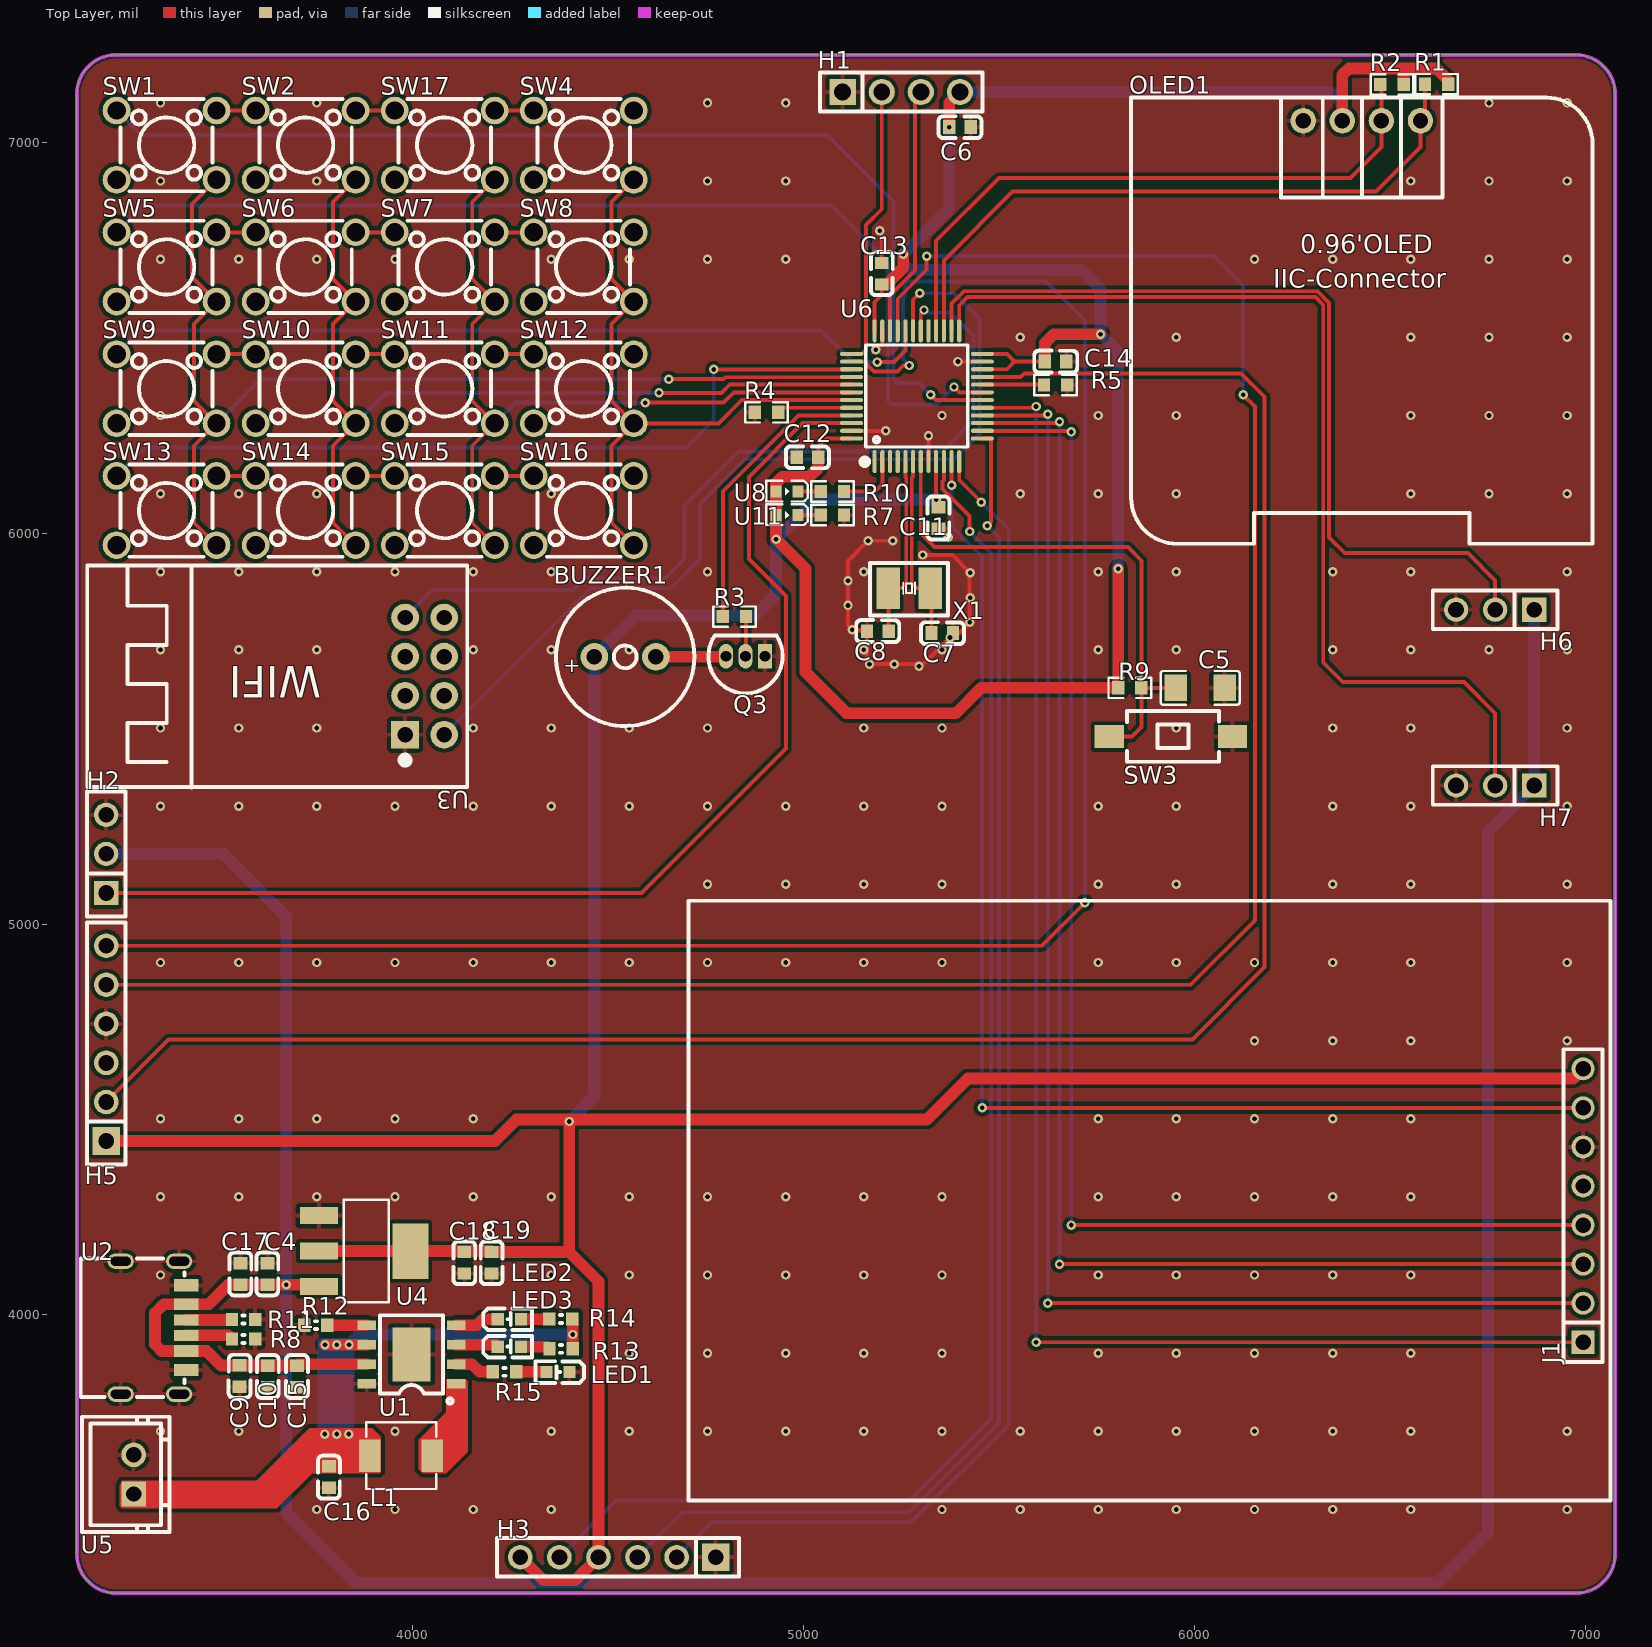
[diagram p0: Top Layer view]
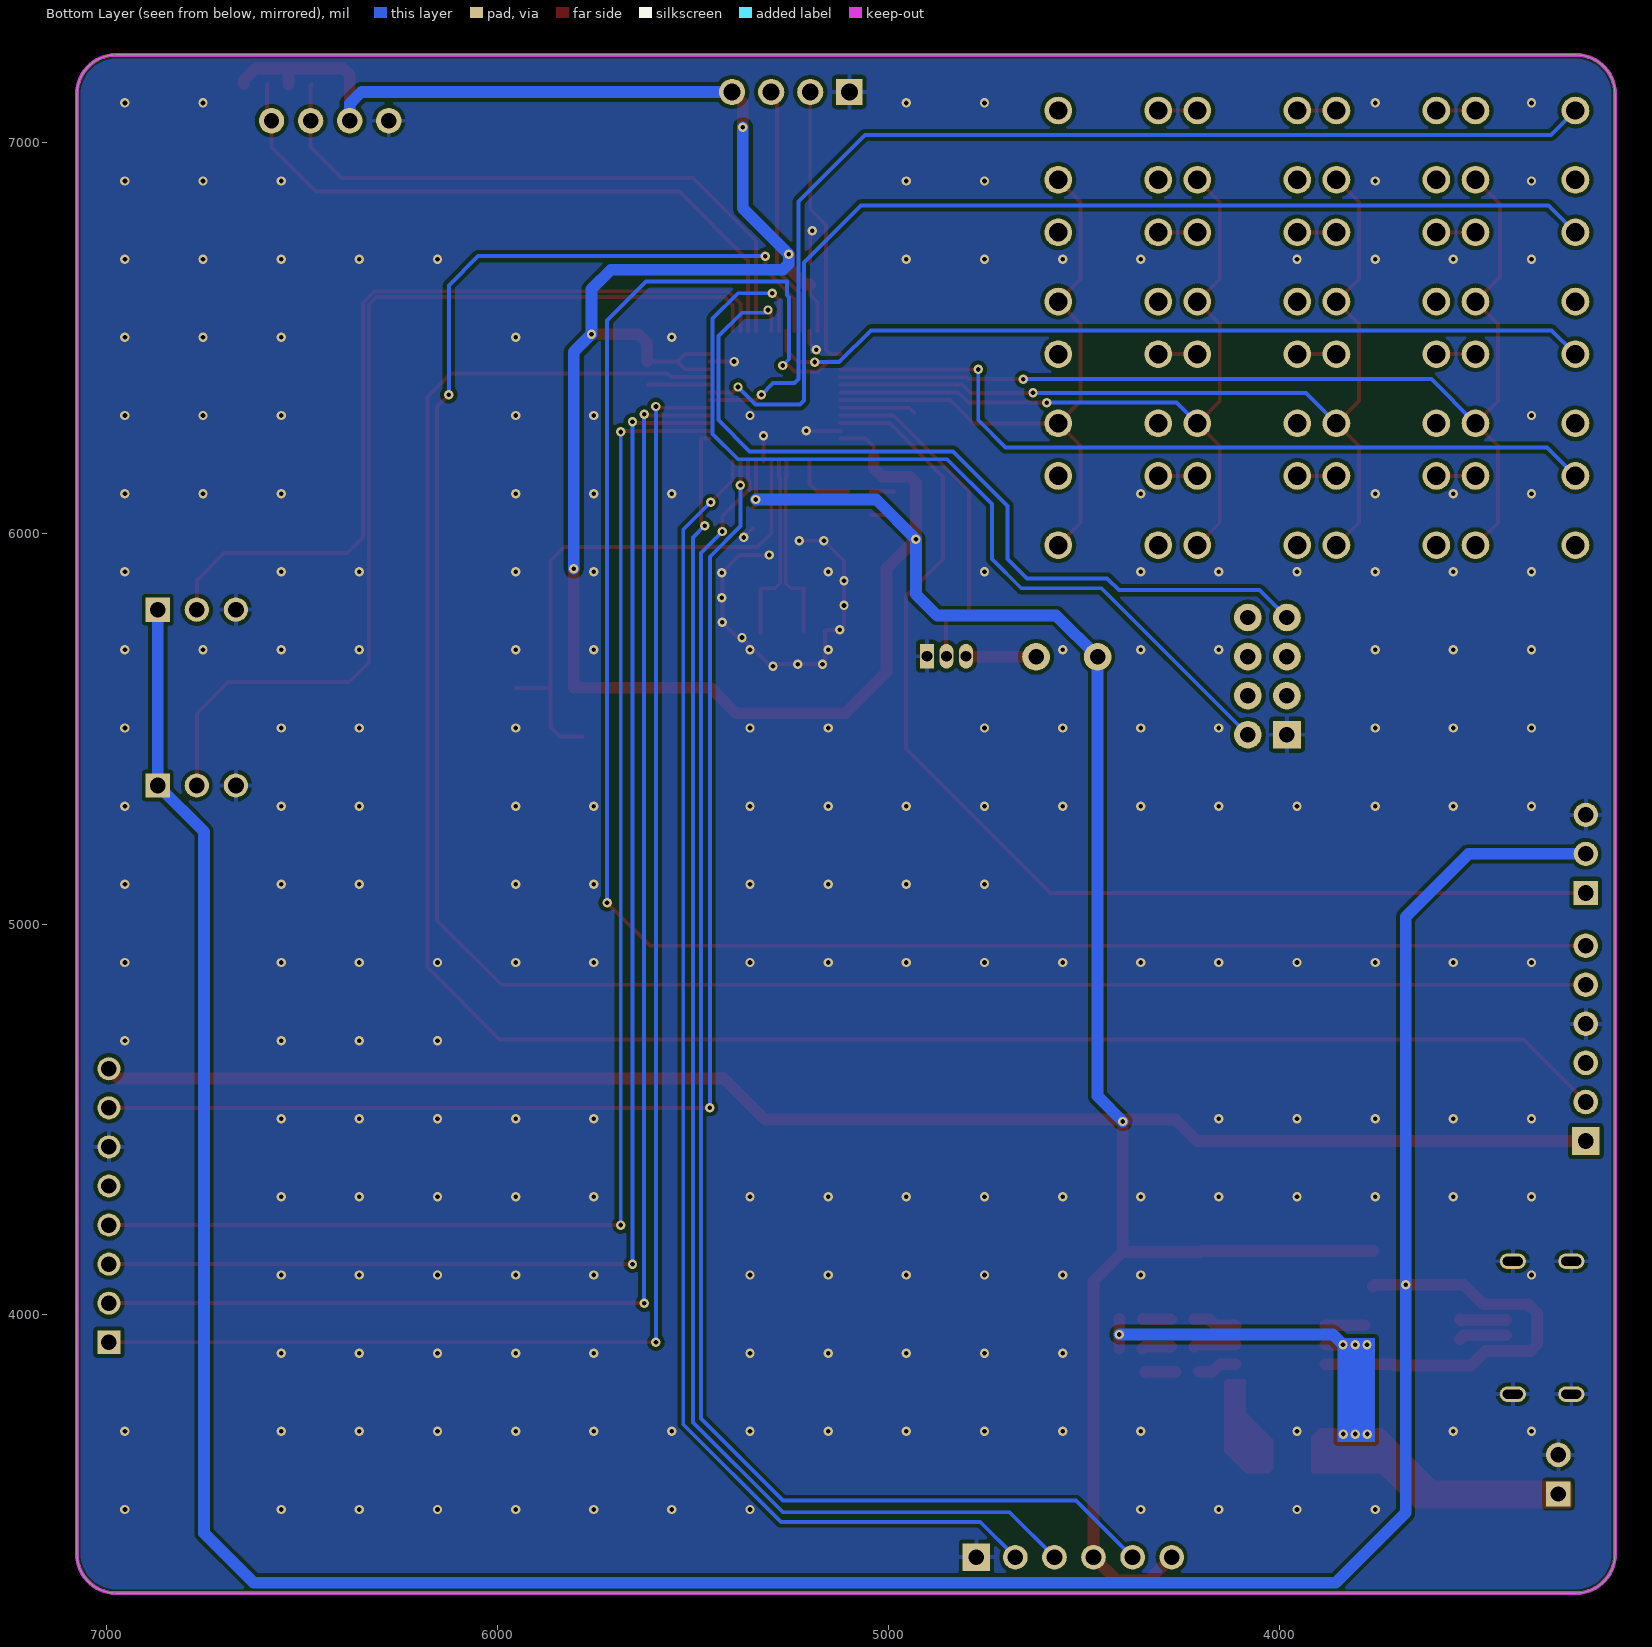
[diagram p1: Bottom Layer view, seen from below]
# Altium PCB MISC51820.pcbdoc
Units mil, origin at the board's own origin, x right, y up, seen from the top; angles counter-clockwise.
Board outline 3937.01 x 3937.01 mil, 2 copper layers (Top Layer, Bottom Layer), stack 62.206 mil thick; 70 components, 71 nets, 263 pads, 270 vias.

## Layer stack, top to bottom
Top Solder Mask Layer: solder mask 0.394, Dk 3.3
Top Layer: signal copper 1.379
Dielectric1: surface 59.449, FR4, Dk 4.5
Bottom Layer: signal copper 1.378
Bottom Solder Mask Layer: solder mask 0.394, Dk 3.3

## Board outline
3240,7225 ccw(c3240,7125) 3140,7125 3140,3387.99 ccw(c3240,3387.99) 3240,3287.99 6977.01,3287.99 ccw(c6977.01,3387.99) 7077.01,3387.99 7077.01,7125 ccw(c6977.01,7125) 6977.01,7225

## Design rules (kind name [scope] priority, off if disabled: settings)
BoardOutlineClearance copperThickness2oz_1 [All] p2 off: genericclearance=7.99 ignorepadtopadclearanceinfootprint=FALSE except(0: Arc-SplitContinuation Track-SplitContinuation SMDPad-SplitContinuation THPad-SplitContinuation Via-SplitContinuation Fill-SplitContinuation Region-SplitContinuation Poly-SplitContinuation Text-SplitContinuation Hole-SplitContinuation; 5.98: Arc-CutoutEdge Track-CutoutEdge SMDPad-CutoutEdge THPad-CutoutEdge Via-CutoutEdge Text-CutoutEdge; 6.9: Hole-OutlineEdge Hole-CutoutEdge; 10: Poly-OutlineEdge Poly-CutoutEdge; 11.81: Arc-OutlineEdge Track-OutlineEdge SMDPad-OutlineEdge THPad-OutlineEdge Via-OutlineEdge Fill-OutlineEdge Region-OutlineEdge Text-OutlineEdge Fill-CutoutEdge Region-CutoutEdge)
BoardOutlineClearance Plane_innerPlane_1 [All] p4 off: genericclearance=4.02 ignorepadtopadclearanceinfootprint=FALSE except(0: Arc-SplitContinuation Track-SplitContinuation SMDPad-SplitContinuation THPad-SplitContinuation Via-SplitContinuation Fill-SplitContinuation Region-SplitContinuation Poly-SplitContinuation Text-SplitContinuation Hole-SplitContinuation; 5.98: Arc-CutoutEdge Track-CutoutEdge SMDPad-CutoutEdge THPad-CutoutEdge Via-CutoutEdge Text-CutoutEdge; 6.9: Hole-OutlineEdge Hole-CutoutEdge; 10: Poly-OutlineEdge Poly-CutoutEdge; 11.81: Arc-OutlineEdge Track-OutlineEdge SMDPad-OutlineEdge THPad-OutlineEdge Via-OutlineEdge Fill-OutlineEdge Region-OutlineEdge Text-OutlineEdge Fill-CutoutEdge Region-CutoutEdge)
BoardOutlineClearance Copper_copperRegion_1 [All] p6 off: genericclearance=4.02 ignorepadtopadclearanceinfootprint=FALSE except(0: Arc-SplitContinuation Track-SplitContinuation SMDPad-SplitContinuation THPad-SplitContinuation Via-SplitContinuation Fill-SplitContinuation Region-SplitContinuation Poly-SplitContinuation Text-SplitContinuation Hole-SplitContinuation; 5.98: Arc-CutoutEdge Track-CutoutEdge SMDPad-CutoutEdge THPad-CutoutEdge Via-CutoutEdge Text-CutoutEdge; 6.9: Hole-OutlineEdge Hole-CutoutEdge; 10: Poly-OutlineEdge Poly-CutoutEdge; 11.81: Arc-OutlineEdge Track-OutlineEdge SMDPad-OutlineEdge THPad-OutlineEdge Via-OutlineEdge Fill-OutlineEdge Region-OutlineEdge Text-OutlineEdge Fill-CutoutEdge Region-CutoutEdge)
BoardOutlineClearance copperThickness1oz_1 [All] p8: genericclearance=4.02 ignorepadtopadclearanceinfootprint=FALSE except(0: Arc-SplitContinuation Track-SplitContinuation SMDPad-SplitContinuation THPad-SplitContinuation Via-SplitContinuation Fill-SplitContinuation Region-SplitContinuation Poly-SplitContinuation Text-SplitContinuation Hole-SplitContinuation; 5.98: Arc-CutoutEdge Track-CutoutEdge SMDPad-CutoutEdge THPad-CutoutEdge Via-CutoutEdge Text-CutoutEdge; 6.9: Hole-OutlineEdge Hole-CutoutEdge; 10: Poly-OutlineEdge Poly-CutoutEdge; 11.81: Arc-OutlineEdge Track-OutlineEdge SMDPad-OutlineEdge THPad-OutlineEdge Via-OutlineEdge Fill-OutlineEdge Region-OutlineEdge Text-OutlineEdge Fill-CutoutEdge Region-CutoutEdge)
Clearance copperThickness2oz [All] p1 off: gap=7.99 ignorepadtopadclearanceinfootprint=FALSE except(5.98: SMDPad-Track SMDPad-SMDPad THPad-Track SMDPad-THPad THPad-THPad Track-Via SMDPad-Via THPad-Via Via-Via Fill-SMDPad Region-SMDPad Fill-THPad Region-THPad Fill-Via Region-Via Fill-Fill Fill-Region Region-Region Arc-Track Arc-SMDPad Arc-THPad Arc-Via Fill-Arc Region-Arc Arc-Arc Text-Track SMDPad-Text Text-THPad Text-Via Fill-Text Region-Text Arc-Text Text-Text; 6.9: Hole-Track Hole-SMDPad Hole-THPad Hole-Via Fill-Hole Region-Hole Hole-Arc Hole-Text; 10: Poly-Track Poly-SMDPad Poly-THPad Poly-Via Poly-Fill Poly-Region Poly-Poly Poly-Arc Poly-Text Poly-Hole; 11.81: Fill-Track Region-Track)
Clearance Plane_innerPlane [All] p3 off: gap=4.02 ignorepadtopadclearanceinfootprint=FALSE except(5.98: SMDPad-Track SMDPad-SMDPad THPad-Track SMDPad-THPad THPad-THPad Track-Via SMDPad-Via THPad-Via Via-Via Fill-SMDPad Region-SMDPad Fill-THPad Region-THPad Fill-Via Region-Via Fill-Fill Fill-Region Region-Region Arc-Track Arc-SMDPad Arc-THPad Arc-Via Fill-Arc Region-Arc Arc-Arc Text-Track SMDPad-Text Text-THPad Text-Via Fill-Text Region-Text Arc-Text Text-Text; 6.9: Hole-Track Hole-SMDPad Hole-THPad Hole-Via Fill-Hole Region-Hole Hole-Arc Hole-Text; 10: Poly-Track Poly-SMDPad Poly-THPad Poly-Via Poly-Fill Poly-Region Poly-Poly Poly-Arc Poly-Text Poly-Hole; 11.81: Fill-Track Region-Track)
Clearance Copper_copperRegion [All] p5 off: gap=4.02 ignorepadtopadclearanceinfootprint=FALSE except(5.98: SMDPad-Track SMDPad-SMDPad THPad-Track SMDPad-THPad THPad-THPad Track-Via SMDPad-Via THPad-Via Via-Via Fill-SMDPad Region-SMDPad Fill-THPad Region-THPad Fill-Via Region-Via Fill-Fill Fill-Region Region-Region Arc-Track Arc-SMDPad Arc-THPad Arc-Via Fill-Arc Region-Arc Arc-Arc Text-Track SMDPad-Text Text-THPad Text-Via Fill-Text Region-Text Arc-Text Text-Text; 6.9: Hole-Track Hole-SMDPad Hole-THPad Hole-Via Fill-Hole Region-Hole Hole-Arc Hole-Text; 10: Poly-Track Poly-SMDPad Poly-THPad Poly-Via Poly-Fill Poly-Region Poly-Poly Poly-Arc Poly-Text Poly-Hole; 11.81: Fill-Track Region-Track)
Clearance copperThickness1oz [All] p7: gap=4.02 ignorepadtopadclearanceinfootprint=FALSE except(5.98: SMDPad-Track SMDPad-SMDPad THPad-Track SMDPad-THPad THPad-THPad Track-Via SMDPad-Via THPad-Via Via-Via Fill-SMDPad Region-SMDPad Fill-THPad Region-THPad Fill-Via Region-Via Fill-Fill Fill-Region Region-Region Arc-Track Arc-SMDPad Arc-THPad Arc-Via Fill-Arc Region-Arc Arc-Arc Text-Track SMDPad-Text Text-THPad Text-Via Fill-Text Region-Text Arc-Text Text-Text; 6.9: Hole-Track Hole-SMDPad Hole-THPad Hole-Via Fill-Hole Region-Hole Hole-Arc Hole-Text; 10: Poly-Track Poly-SMDPad Poly-THPad Poly-Via Poly-Fill Poly-Region Poly-Poly Poly-Arc Poly-Text Poly-Hole; 11.81: Fill-Track Region-Track)
DiffPairsRouting differentialPair [All] p1: maxlimit=6 minlimit=6 mostfreqgap=6 toplayer_minwidth=5 toplayer_prefwidth=10 toplayer_maxwidth=100 toplayer_mingap=6 toplayer_prefgap=6 toplayer_maxgap=6 bottomlayer_minwidth=5 bottomlayer_prefwidth=10 bottomlayer_maxwidth=100 bottomlayer_mingap=6 bottomlayer_prefgap=6 bottomlayer_maxgap=6 maxuncoupledlength=10
HoleToHoleClearance otherClearance [All] p1: gap=11.81 allowstackedmicrovias=TRUE
Length netLength [All] p1: minlimit=0 maxlimit=0
PasteMaskExpansion pasteMaskExpansion [All] p1: expansion=0
PlaneConnect innerPlane [All] p1: planeconnectstyle=Relief reliefexpansion=20 reliefentries=4 reliefconductorwidth=10 reliefairgap=10
PolygonConnect copperRegion [All] p1: connectstyle=Relief reliefconductorwidth=10 reliefentries=4 polygonreliefangle="90 Angle" airgapwidth=10 via.connectstyle=Relief via.reliefconductorwidth=10 via.reliefentries=4 via.polygonreliefangle="90 Angle" via.airgapwidth=10
RoutingVias viaSize [All] p1: holewidth=12.01 width=24.02 viastyle="Through Hole" minholewidth=11.81 minwidth=19.68 maxholewidth=248.03 maxwidth=393.7
SolderMaskExpansion solderMaskExpansion [IsVia] p1: expansion=-1000 istentingtop=TRUE
SolderMaskExpansion solderMaskExpansion [All] p2: expansion=2 istentingtop=FALSE
Width copperThickness2oz_2 [All] p1 off: maxlimit=100 minlimit=8 preferedwidth=10
Width copperThickness1oz_2 [All] p2: maxlimit=100 minlimit=5 preferedwidth=10

## Components (designator, comment, footprint, x,y, rotation, side; value= is the part's Value field where it differs from the comment)
BUZZER1 "2.7kHz" BUZ-TH_BD9.0-P4.00-D0.6-FD 4543.28,5684.32 r0 top
C4 "10uF" C0603 3627.51,4104.85 r270 top
C5 "100uF" C1206 6015,5605 r180 top
C6 "100nF" C0603 5400,7040 r180 top
C7 "20pF" C0603 5355,5745 r180 top
C8 "20pF" C0603 5190,5750 r0 top
C9 "22uF" C0603 3556.59,3843.41 r90 top
C10 "22uF" C0603 3628.64,3842.73 r90 top
C11 "100nF" C0603 5345,6040 r90 top
C12 "100nF" C0603 5010,6195 r0 top
C13 "100nF" C0603 5200,6665 r270 top
C14 "100nF" C0603 5645,6440 r180 top
C15 "22uF" C0603 3703.38,3842.73 r90 top
C16 "22uF" C0603 3785,3585 r90 top
C17 "100nF" C0603 3558.38,4104.85 r270 top
C18 "10uF" C0603 4131.59,4133.41 r90 top
C19 "100nF" C0603 4201.59,4133.41 r90 top
H1 "" HDR-TH_4P-P2.54-V-F 5250,7130 r0 top
H2 "" HDR-TH_3P-P2.54-V-F 3215,5180 r90 top
H3 "" HDR-TH_6P-P2.54-V-F 4525,3380 r180 top
H5 "" HDR-TH_6P-P2.54-V-F 3215,4695 r90 top
H6 "" HDR-TH_3P-P2.54-V-F 6770,5805 r180 top
H7 "" HDR-TH_3P-P2.54-V-F 6770,5355 r180 top
J1 "" HDR-TH_8P-P2.54-V-M 6995,4280 r90 top
L1 "2.2uH" IND-SMD_L4.4-W4.2 3970,3640 r180 top
LED1 "Battery" LED0603_L1.6-W0.8-RD_BLUE 4371.39,3853.75 r180 top
LED2 "Discharge" LED0603_L1.6-W0.8-RD_BLUE 4247.02,3988.81 r0 top
LED3 "Charge" LED0603_L1.6-W0.8-RD_BLUE 4247.02,3918.81 r0 top
OLED1 "" 0.96OLED_4P 6428.8,7056.43 r0 top
Q3 "" S8050_TO_92 4851.43,5685.89 r180 top
R1 "5.1K" R0603 6620,7150 r0 top
R2 "5.1K" R0603 6505.98,7149.32 r0 top
R3 "1K" R0603 4822.85,5787.32 r180 top
R4 "10kΩ" R0603 4905,6310 r0 top
R5 "10kΩ" R0603 5645,6380 r180 top
R7 "510Ω" R0603 5073.8,6047.22 r0 top
R8 "5.1K" R0603-NSK 3566.59,3938.41 r180 top
R9 "1kΩ" R0603 5835,5605 r180 top
R10 "510Ω" R0603 5073.8,6107.52 r0 top
R11 "5.1K" R0603-NSK 3566.59,3988.41 r180 top
R12 "56K" R0603-NSK 3751.59,3973.91 r180 top
R13 "5.1K" R0603-NSK 4379.2,3913.13 r180 top
R14 "5.1K" R0603-NSK 4378.67,3989.49 r180 top
R15 "5.1K" R0603-NSK 4234.52,3854.37 r180 top
SW1 "KH-6X6X6H-TJ" SW-TH_4P-L6.0-W6.0-P4.50-LS6.5 3369.4,6994.04 r0 top
SW2 "KH-6X6X6H-TJ" SW-TH_4P-L6.0-W6.0-P4.50-LS6.5 3725.37,6994.04 r0 top
SW3 "TS-1101-C-W" SW-SMD_L6.0-W3.3-LS8.0 5940,5480 r180 top
SW4 "KH-6X6X6H-TJ" SW-TH_4P-L6.0-W6.0-P4.50-LS6.5 4437.3,6994.04 r0 top
SW5 "KH-6X6X6H-TJ" SW-TH_4P-L6.0-W6.0-P4.50-LS6.5 3369.4,6682.26 r0 top
SW6 "KH-6X6X6H-TJ" SW-TH_4P-L6.0-W6.0-P4.50-LS6.5 3725.37,6682.26 r0 top
SW7 "KH-6X6X6H-TJ" SW-TH_4P-L6.0-W6.0-P4.50-LS6.5 4081.33,6682.26 r0 top
SW8 "KH-6X6X6H-TJ" SW-TH_4P-L6.0-W6.0-P4.50-LS6.5 4437.3,6682.26 r0 top
SW9 "KH-6X6X6H-TJ" SW-TH_4P-L6.0-W6.0-P4.50-LS6.5 3369.4,6370.49 r0 top
SW10 "KH-6X6X6H-TJ" SW-TH_4P-L6.0-W6.0-P4.50-LS6.5 3725.37,6370.49 r0 top
SW11 "KH-6X6X6H-TJ" SW-TH_4P-L6.0-W6.0-P4.50-LS6.5 4081.33,6370.49 r0 top
SW12 "KH-6X6X6H-TJ" SW-TH_4P-L6.0-W6.0-P4.50-LS6.5 4437.3,6370.49 r0 top
SW13 "KH-6X6X6H-TJ" SW-TH_4P-L6.0-W6.0-P4.50-LS6.5 3369.4,6058.72 r0 top
SW14 "KH-6X6X6H-TJ" SW-TH_4P-L6.0-W6.0-P4.50-LS6.5 3725.37,6058.72 r0 top
SW15 "KH-6X6X6H-TJ" SW-TH_4P-L6.0-W6.0-P4.50-LS6.5 4081.33,6058.72 r0 top
SW16 "KH-6X6X6H-TJ" SW-TH_4P-L6.0-W6.0-P4.50-LS6.5 4437.3,6058.72 r0 top
SW17 "KH-6X6X6H-TJ" SW-TH_4P-L6.0-W6.0-P4.50-LS6.5 4081.33,6994.04 r0 top
U1 "ETA9742" ESOP-8_L4.9-W3.9-P1.27-LS6.0-BL-EP 3996.39,3898.81 r90 top
U2 "YTC-TC6-268" TYPE-C-SMD_YIYUAN_YTC-TC6-268 3335.87,3967.32 r270 top
U3 "2.4GHz" WIFIM-TH_8P-L24.7-W14.4-P2.54 4030,5635 r180 top
U4 "AMS1117-3.3" SOT-223-3_L6.5-W3.4-P2.30-LS7.0-BR 3876.59,4163.41 r180 top
U5 "_x001F_XH2.54-2P" CONN-TH_2P-P2.54-V 3285.24,3591.72 r90 top
U6 "STM32F103C8T6" LQFP-48_L7.0-W7.0-P0.50-LS9.0-BL 5290.06,6351.43 r0 top
U8 "42-51/GHC-YW2X2K/3T" LED-SMD_L1.6-W0.8-FD_GREEN-1 4957.67,6107.52 r0 top
U11 "42-51/GHC-YW2X2K/3T" LED-SMD_L1.6-W0.8-FD_GREEN-1 4957.67,6047.22 r0 top
X1 "8MHz" CRYSTAL-SMD_L3.2-W2.5_3225-8MHZ 5270,5860 r180 top

## Footprints (in the part's own frame and the unit in brackets; to place one, negate y for a bottom-side part, rotate by r counter-clockwise, add the part's x,y. Pads: shape width x height; smd on the part's side, far side on the other; paste and mask are expansions set on the pad)
0.96OLED_4P [mm]
  round 1.65 hole 1 copper offset 0,0: 1(-3.81,-0.001) 2(-1.27,0.002) 3(1.27,0.002) 4(3.81,0.002)
  silkscreen extent -15,-27.5 15,1.5
BUZ-TH_BD9.0-P4.00-D0.6-FD [mm]
  round 1.8 hole 1: 1(-2,0) 2(2,0)
  silkscreen extent -4.5,-4.5 4.5,4.5
C0603 [mm]
  rect 0.8x0.9 smd: 1(-0.7,0) 2(0.7,0)
  silkscreen extent -1.39,-0.71 1.39,0.71
C1206 [mm]
  rect 1.485x1.728 smd paste-100 mask+0.051: 1(-1.593,0) 2(1.593,0)
  silkscreen extent -2.56,-1.09 2.56,1.09
CONN-TH_2P-P2.54-V [mm]
  rect 1.6x1.6 hole 1: 1(-1.27,0)
  round 1.6 hole 1: 2(1.27,0)
  silkscreen extent -3.75,-2.34 3.75,3.36
CRYSTAL-SMD_L3.2-W2.5_3225-8MHZ [mil]
  rect 60x106.3 smd paste+0 mask+1.97: 1(-53.62,0) 2(53.62,0)
  silkscreen extent -100,-65 100,70
ESOP-8_L4.9-W3.9-P1.27-LS6.0-BL-EP [mm]
  rect 0.6x1.2 smd paste+0 mask+0.051: 1(-1.905,-2.908) 2(-0.635,-2.908) 3(0.635,-2.908) 4(1.905,-2.908) 5(1.905,2.908) 6(0.635,2.908) 7(-0.635,2.908) 8(-1.905,2.908)
  rect 3.5x2.5 smd paste+0 mask+0.051: 9(0,0)
  silkscreen extent -3.2,-2.67 2.55,2.05
HDR-TH_3P-P2.54-V-F [mil]
  rect 62x62 hole 40.16: 1(-100,0)
  round 62 hole 40.16: 2(0,0) 3(100,0)
  silkscreen extent -160,-49 160,49
HDR-TH_4P-P2.54-V-F [mm]
  rect 1.7x1.7 hole 1.1: 1(-3.81,0)
  round 1.7 hole 1.1: 2(-1.27,0) 3(1.27,0) 4(3.81,0)
  silkscreen extent -5.29,-1.27 5.29,1.27
HDR-TH_6P-P2.54-V-F [mm]
  rect 1.8x1.8 hole 1.02: 1(-6.35,0)
  round 1.6 hole 1.02: 2(-3.81,0) 3(-1.27,0) 4(1.27,0) 5(3.81,0) 6(6.35,0)
  silkscreen extent -7.87,-1.25 7.87,1.25
HDR-TH_8P-P2.54-V-M [mm]
  rect 1.5x1.5 hole 1: 1(-8.89,0)
  round 1.5 hole 1: 2(-6.35,0) 3(-3.81,0) 4(-1.27,0) 5(1.27,0) 6(3.81,0) 7(6.35,0) 8(8.89,0)
  silkscreen extent -10.16,-1.27 10.16,1.27
IND-SMD_L4.4-W4.2 [mm]
  rect 1.4x2.12 smd paste+0 mask+0.051: 1(2.028,0) 2(-2.028,0)
  silkscreen extent -2.28,-2.18 2.28,2.18
LED0603_L1.6-W0.8-RD_BLUE [mm]
  rect 0.8x0.8 smd: 1(-0.75,0) 2(0.75,0)
  silkscreen extent -1.7,-0.7 1.47,0.7
LED-SMD_L1.6-W0.8-FD_GREEN-1 [mm]
  rect 0.7x0.8 smd: 1(-0.715,0) 2(0.715,0)
  silkscreen extent -1.35,-0.65 1.35,0.7
LQFP-48_L7.0-W7.0-P0.50-LS9.0-BL [mm]
  oval 0.27x1.5 smd paste+0 mask+0.05: 1(-2.75,-4.25) 2(-2.25,-4.25) 3(-1.75,-4.25) 4(-1.25,-4.25) 5(-0.75,-4.25) 6(-0.25,-4.25) 7(0.25,-4.25) 8(0.75,-4.25) 9(1.25,-4.25) 10(1.75,-4.25) 11(2.25,-4.25) 12(2.75,-4.25) 25(2.75,4.25) 26(2.25,4.25) 27(1.75,4.25) 28(1.25,4.25) 29(0.75,4.25) 30(0.25,4.25) 31(-0.25,4.25) 32(-0.75,4.25) 33(-1.25,4.25) 34(-1.75,4.25) 35(-2.25,4.25) 36(-2.75,4.25)
  oval 1.5x0.27 smd paste+0 mask+0.05: 13(4.25,-2.75) 14(4.25,-2.25) 15(4.25,-1.75) 16(4.25,-1.25) 17(4.25,-0.75) 18(4.25,-0.25) 19(4.25,0.25) 20(4.25,0.75) 21(4.25,1.25) 22(4.25,1.75) 23(4.25,2.25) 24(4.25,2.75) 37(-4.25,2.75) 38(-4.25,2.25) 39(-4.25,1.75) 40(-4.25,1.25) 41(-4.25,0.75) 42(-4.25,0.25) 43(-4.25,-0.25) 44(-4.25,-0.75) 45(-4.25,-1.25) 46(-4.25,-1.75) 47(-4.25,-2.25) 48(-4.25,-2.75)
  silkscreen extent -3.59,-4.46 3.3,3.34
R0603 [mil]
  rect 31.75x34.02 smd paste-3937.01 mask+2: 1(-29.66,0) 2(29.66,0)
  silkscreen extent -55,-26 55,26
R0603-NSK [mil]
  rect 31.75x34.02 smd paste-3937.01 mask+2: 1(-29.65,0) 2(29.66,0)
  silkscreen extent -3,-10 3,10
S8050_TO_92 [mil]
  rect 35.4x63 hole 27.6 paste+0 mask+2: 1(-50,0)
  oval 35.4x63 hole 27.6 paste+0 mask+2: 2(0,0) 3(50,0)
  silkscreen extent -95,-53 95,95
SOT-223-3_L6.5-W3.4-P2.30-LS7.0-BR [mm]
  rect 2.5x1.1 smd: 1(2.97,-2.3) 2(2.97,0) 3(2.97,2.3)
  rect 2.34x3.6 smd: 4(-2.97,0)
  silkscreen extent -1.57,-3.33 1.37,3.33
SW-SMD_L6.0-W3.3-LS8.0 [mm]
  rect 1.9x1.5 smd: 1(-4,0) 2(4,0)
  silkscreen extent -3.14,-1.67 2.86,1.63
SW-TH_4P-L6.0-W6.0-P4.50-LS6.5 [mm]
  round 1.8 hole 1.2: 1(-3.25,2.25) 2(3.25,2.25) 3(-3.25,-2.25) 4(3.25,-2.25)
  silkscreen extent -3,-3 3,3
TYPE-C-SMD_YIYUAN_YTC-TC6-268 [mm]
  oval 1x1.7 hole 0.6 slot 1.3 at 90 deg paste+0 mask+0.05: 1(-4.32,1.676) 2(4.32,1.676) 3(4.32,-2.125) 4(-4.32,-2.125)
  rect 0.7x1.6 smd paste-100 mask+0.05: A5(-0.5,2.125) B5(0.5,2.125)
  rect 0.76x1.6 smd paste-100 mask+0.05: A9(1.52,2.125) B9(-1.52,2.125)
  rect 0.8x1.6 smd paste-100 mask+0.05: A12(2.75,2.125) B12(-2.75,2.125)
  silkscreen extent -4.5,-4.72 4.5,2.03
WIFIM-TH_8P-L24.7-W14.4-P2.54 [mm]
  rect 1.8x1.8 hole 1 paste+0 mask+0.05: 1(1.27,3.81)
  round 1.8 hole 1 paste+0 mask+0.05: 2(1.27,1.27) 3(1.27,-1.27) 4(1.27,-3.81) 5(-1.27,3.81) 6(-1.27,1.27) 7(-1.27,-1.27) 8(-1.27,-3.81)
  silkscreen extent -2.77,-7.19 21.93,7.24

## Via types
v1: diameter 24.02, hole 12, Top Layer to Bottom Layer, 270 vias

## Nets (pads, with @x,y where several pads share a name; then routed paths per layer and width w, separated by ;. In a path a pad name is that pad's centre, name@x,y a point inside that pad or via, vN(x,y) a via of type N, cw(c..) or ccw(c..) an arc to the next point about the centre after c; other vN are vias at no path point)
$1N1877: BUZZER1.2 Q3.3 | length 180.1
  Top Layer w30: BUZZER1.2 4799.86,5684.32 Q3.3
$1N2018: Q3.2 R3.1 | length 101.9
  Top Layer w10: Q3.2 4852.51,5686.98 R3.1
$1N5108: R7.1 U11.2 | length 58.3
  Top Layer w10: U11.2 R7.1
$1N5109: R10.1 U8.2 | length 58.3
  Top Layer w10: U8.2 R10.1
$1N5277: SW9.2 SW10.1 | length 100.1
  Top Layer w10: SW9.2 SW10.1
$1N5278: SW13.2 SW14.1 | length 100.1
  Top Layer w10: SW13.2 SW14.1
$1N5279: SW15.2 SW16.1 | length 100.1
  Top Layer w10: SW15.2 SW16.1@4309.35,6147.3
$1N5280: SW14.2 SW15.1 | length 100.1
  Top Layer w10: SW14.2 SW15.1
$1N5281: SW11.2 SW12.1 | length 100.1
  Top Layer w10: SW11.2 SW12.1@4309.35,6459.07
$1N5282: SW10.2 SW11.1 | length 100.1
  Top Layer w10: SW10.2 SW11.1
$1N5283: SW7.2 SW8.1 | length 100.1
  Top Layer w10: SW7.2 SW8.1@4309.35,6770.84
$1N5284: SW5.2 SW6.1 | length 100.1
  Top Layer w10: SW5.2 SW6.1
$1N5285: SW6.2 SW7.1 | length 100.1
  Top Layer w10: SW6.2 SW7.1
$1N5286: SW1.2 SW2.1 | length 100.1
  Top Layer w10: SW1.2 SW2.1
$1N5287: SW2.2 SW17.1 | length 100.1
  Top Layer w10: SW2.2 SW17.1
$1N5288: SW4.1 SW17.2 | length 100.1
  Top Layer w10: SW17.2 SW4.1@4309.35,7082.62
$1N5308: LED3.2 R13.2 | length 75.3
  Top Layer w30: LED3.2 4343.87,3918.81 R13.2
$1N5310: LED1.2 R15.1 | length 77.9
  Top Layer w30: R15.1 4341.24,3854.37 LED1.2
$1N5311: LED2.2 R14.2 | length 72.8
  Top Layer w30: LED2.2 4348.33,3988.81 R14.2
$1N5312: LED2.1 U1.4 | length 112.8
  Top Layer w30: U1.4 4163.81,3973.81 4178.81,3988.81 LED2.1
$1N5313: R8.2 U2.B5 | length 121.2
  Top Layer w30: U2.B5 3527.72,3947.63 R8.2
$1N5314: R11.2 U2.A5 | length 118
  Top Layer w30: U2.A5 3535.52,3987 R11.2
$1N5317: LED3.1 U1.3 | length 108.7
  Top Layer w30: U1.3 4212.49,3923.81 LED3.1
$1N5319: R15.2 U1.2 | length 102
  Top Layer w30: U1.2 4151.19,3873.81 4170.63,3854.37 R15.2
$1N5320: R12.1 U1.5 | length 100.7
  Top Layer w30: R12.1 3881.79,3973.91 U1.5
$1N5322: L1.2 U1.1
+3.3V: U3.8
+5V: C4.2 C9.2 C10.2 C15.2 C17.2 H2.2 H6.1 H7.1 U1.7 U2.A9 U2.B9 U4.3 | length 8764.9
  Top Layer w30: U4.3 3755.24,4077.29 v1(3676,4077.29) C4.2 C17.2 3527.29,4077.29 3477.16,4027.16 U2.B9 3362.16,4027.16 3340,4005 3340,3925 3357.53,3907.47 U2.A9 3472.53,3907.47 3509.71,3870.29 C10.2 C15.2 3706.9,3873.81 U1.7
  Bottom Layer w30: H2.2 3515,5180 3676,5019 v1(3676,4077.29) 3676,3494 3855.2,3314.8 6624.8,3314.8 6751.53,3441.53 6751.53,5236.53 H7.1 H6.1
BAT: C16.2 L1.1 R13.1 R14.1 U1.6 U5.1 | length 766.9
  Top Layer w30: v1(3775,3923.81) v1(3805.38,3923.81) v1(3836.32,3923.81) U1.6 ; R14.1 4408.85,3988.96 v1(4408.85,3950) R13.1
  Bottom Layer w30: v1(3836.32,3923.81) 3862.51,3950 v1(4408.85,3950)
  other v1: 3774.34,3695 3804.73,3695 3835.66,3695
BEEP: R3.2 U6.45 | length 730.8
  Top Layer w10: R3.2 4793.19,6108.19 4987.22,6302.22 U6.45
BOOT0: R4.2 U6.44 | length 193
  Top Layer w10: R4.2 4946.56,6321.9 U6.44
BOOT1: R5.2 U6.20 | length 158.4
  Top Layer w10: U6.20 5614.38,6380.96 R5.2
CLK: H1.2 U6.37 | length 718.1
  Top Layer w10: U6.37 5149.7,6459.7 5160,6470 5160,6790 5200,6830 H1.2
DHT11: H6.2 U6.26 | length 2207.2
  Top Layer w10: U6.26 5378.64,6588.64 5410,6620 6315,6620 6345,6590 6345,5990 6385,5950 6700,5950 6770,5880 H6.2
DIO: H1.3 U6.34 | length 643.9
  Top Layer w10: U6.34 5221.16,6609.6 5285,6673.44 5285,7115 H1.3
GND: C4.1 C5.1 C6.1 C7.1 C8.1 C9.1 C10.1 C11.1 C12.1 C13.1 C14.1 C15.1 C16.1 C17.1 C18.1 C19.1 H1.1 H2.3 H3.1 H5.4 H6.3 H7.3 J1.6 LED1.1 OLED1.1 Q3.1 R4.1 R5.1 R7.2 R8.1 R11.1 R12.2 SW3.1 U1.8 U1.9 U2.1 U2.2 U2.3 U2.4 U2.A12 U2.B12 U3.1 U4.1 U5.2 U6.8 U6.23 U6.35 U6.47 | length 1406.2
  Top Layer w10: U6.47 v1(5210,6262.85) ; v1(5185,6470) 5201.48,6486.48 U6.35 ; v1(5195,6775) 5200,6770 C13.1 ; v1(5228.39,5981.38) v1(5165,5981.38) 5113.62,5930 v1(5113.62,5879.29) v1(5113.62,5815.91) 5113.62,5764.28 v1(5124.45,5753.45) 5158.99,5753.45 C8.1 5162.44,5671.95 v1(5168.72,5665.67) v1(5232.1,5665.67) 5290.06,5665.67 v1(5295.27,5660.46) 5301.64,5660.46 v1(5374.81,5733.62) 5385.93,5733.62 v1(5424.84,5772.54) 5424.84,5897.75 v1(5426.38,5899.29) 5380.67,5945 v1(5305,5945) ; U6.8 v1(5319.59,6250) ; C11.1 5347.99,6012.44 v1(5370.44,5989.99) ; v1(5395,6440.01) U6.23
  other v1: 3754.1,3502.09 3954.1,3502.09 4154.1,3502.09 4354.1,3502.09 5354.1,3502.09 5554.1,3502.09 5754.1,3502.09 5954.1,3502.09 6154.1,3502.09 6354.1,3502.09 6554.1,3502.09 6954.1,3502.09 3354.1,3702.09 3554.1,3702.09 3954.1,3702.09 4354.1,3702.09 4554.1,3702.09 4754.1,3702.09 4954.1,3702.09 5154.1,3702.09 5354.1,3702.09 5554.1,3702.09 5754.1,3702.09 5954.1,3702.09 6154.1,3702.09 6354.1,3702.09 6554.1,3702.09 6954.1,3702.09 4554.1,3902.09 4754.1,3902.09 4954.1,3902.09 5154.1,3902.09 5354.1,3902.09 5754.1,3902.09 5954.1,3902.09 6154.1,3902.09 6354.1,3902.09 6554.1,3902.09 3354.1,4102.09 4354.1,4102.09 4554.1,4102.09 4754.1,4102.09 4954.1,4102.09 5154.1,4102.09 5354.1,4102.09 5754.1,4102.09 5954.1,4102.09 6154.1,4102.09 6354.1,4102.09 6554.1,4102.09 3354.1,4302.09 3554.1,4302.09 3754.1,4302.09 3954.1,4302.09 4154.1,4302.09 4354.1,4302.09 4554.1,4302.09 4754.1,4302.09 4954.1,4302.09 5154.1,4302.09 5354.1,4302.09 5754.1,4302.09 5954.1,4302.09 6154.1,4302.09 6354.1,4302.09 6554.1,4302.09 3354.1,4502.09 3554.1,4502.09 3754.1,4502.09 3954.1,4502.09 4154.1,4502.09 5754.1,4502.09 5954.1,4502.09 6154.1,4502.09 6354.1,4502.09 6554.1,4502.09 6154.1,4702.09 6354.1,4702.09 6554.1,4702.09 6954.1,4702.09 3354.1,4902.09 3554.1,4902.09 3754.1,4902.09 3954.1,4902.09 4154.1,4902.09 4354.1,4902.09 4554.1,4902.09 4754.1,4902.09 4954.1,4902.09 5154.1,4902.09 5354.1,4902.09 5754.1,4902.09 5954.1,4902.09 6154.1,4902.09 6354.1,4902.09 6554.1,4902.09 6954.1,4902.09 4754.1,5102.09 4954.1,5102.09 5154.1,5102.09 5354.1,5102.09 5754.1,5102.09 5954.1,5102.09 6354.1,5102.09 6554.1,5102.09 6954.1,5102.09 3354.1,5302.09 3554.1,5302.09 3754.1,5302.09 3954.1,5302.09 4154.1,5302.09 4354.1,5302.09 4554.1,5302.09 4754.1,5302.09 4954.1,5302.09 5154.1,5302.09 5354.1,5302.09 5754.1,5302.09 5954.1,5302.09 6354.1,5302.09 6554.1,5302.09 6954.1,5302.09 3354.1,5502.09 3554.1,5502.09 3754.1,5502.09 4154.1,5502.09 4354.1,5502.09 4554.1,5502.09 4754.1,5502.09 5154.1,5502.09 5354.1,5502.09 5954.1,5502.09 6354.1,5502.09 6554.1,5502.09 6954.1,5502.09 3354.1,5702.09 3554.1,5702.09 3754.1,5702.09 4154.1,5702.09 4354.1,5702.09 4554.1,5702.09 5154.1,5702.09 5354.1,5702.09 5754.1,5702.09 5954.1,5702.09 6354.1,5702.09 6554.1,5702.09 6754.1,5702.09 6954.1,5702.09 5426.38,5835.9 3354.1,5902.09 3554.1,5902.09 3754.1,5902.09 3954.1,5902.09 4154.1,5902.09 4354.1,5902.09 4754.1,5902.09 5154.1,5902.09 5754.1,5902.09 5954.1,5902.09 6354.1,5902.09 6554.1,5902.09 6954.1,5902.09 3354.1,6102.09 3554.1,6102.09 3754.1,6102.09 4354.1,6102.09 5554.1,6102.09 5754.1,6102.09 5954.1,6102.09 6554.1,6102.09 6754.1,6102.09 6954.1,6102.09 3354.1,6302.09 5354.1,6302.09 5754.1,6302.09 5954.1,6302.09 6554.1,6302.09 6754.1,6302.09 6954.1,6302.09 5554.1,6502.09 5954.1,6502.09 6554.1,6502.09 6754.1,6502.09 6954.1,6502.09 3354.1,6702.09 3554.1,6702.09 3754.1,6702.09 3954.1,6702.09 4354.1,6702.09 4554.1,6702.09 4754.1,6702.09 4954.1,6702.09 6154.1,6702.09 6354.1,6702.09 6554.1,6702.09 6754.1,6702.09 6954.1,6702.09 3354.1,6902.09 3754.1,6902.09 4754.1,6902.09 4954.1,6902.09 6554.1,6902.09 6754.1,6902.09 6954.1,6902.09 3354.1,7102.09 3754.1,7102.09 4754.1,7102.09 4954.1,7102.09 6754.1,7102.09 6954.1,7102.09
HCSR501: H7.2 U6.25 | length 2607.4
  Top Layer w10: U6.25 5398.33,6583.33 5420,6605 6310,6605 6330,6585 6330,5670 6380,5620 6690,5620 6770,5540 H7.2
MFR_MISO: J1.4 U6.14 | length 3568.8
  Top Layer w10: U6.14 5682.15,6262.85 v1(5685,6260) ; v1(5685,4230) J1.4
  Bottom Layer w10: v1(5685,4230) v1(5685,6260)
MFR_MOSI: J1.3 U6.15 | length 3694.8
  Top Layer w10: U6.15 5651.69,6282.53 v1(5655,6285.84) ; v1(5655,4130) J1.3
  Bottom Layer w10: v1(5655,4130) v1(5655,6285.84)
MFR_RST: J1.7 U6.11 | length 3224.6
  Top Layer w10: U6.11 5378.64,6123.85 v1(5378.74,6123.74) ; v1(5457.01,4530) J1.7
  Bottom Layer w10: v1(5378.74,6123.74) 5378.74,6018.74 5457.01,5940.48 v1(5457.01,4530)
MFR_SCK: J1.2 U6.16 | length 3814.5
  Top Layer w10: U6.16 5621.7,6302.22 v1(5625,6305.52) ; v1(5625,4030) J1.2
  Bottom Layer w10: v1(5625,4030) v1(5625,6305.52)
MFR_SDA: J1.1 U6.17 | length 3934.2
  Top Layer w10: U6.17 5591.69,6321.9 v1(5595,6325.21) ; v1(5595,3930) J1.1
  Bottom Layer w10: v1(5595,3930) v1(5595,6325.21)
OLED_SCL: OLED1.3 R2.1 U6.28 | length 1630.8
  Top Layer w10: U6.28 5339.27,6749.27 5500,6910 6400,6910 6478.8,6988.8 OLED1.3 6478.8,7146.84 R2.1
OLED_SDA: OLED1.4 R1.1 U6.27 | length 1686.1
  Top Layer w10: U6.27 5358.96,6698.96 5535,6875 6465,6875 6578.8,6988.8 OLED1.4 6590.34,7068.02 R1.1
OSC32-IN: U6.3
OSC32-OUT: U6.4
OSC-IN: C8.2 U6.5 X1.2 | length 474.5
  Top Layer w10: C8.2 5217.56,5858.82 X1.2 5250,5860 5262.81,5872.81 5262.81,6142.19 5260.53,6144.47 U6.5
OSC-OUT: C7.2 U6.6 X1.1 | length 481.2
  Top Layer w10: U6.6 5280.22,6145.22 5276.82,6141.82 5276.82,5873.18 5290,5860 X1.1 5327.44,5856.18 C7.2
PA0: H3.5 U6.10 | length 3754
  Top Layer w10: U6.10 5358.96,6136.47 5355.75,6133.27 5355.75,6114.22 5425,6045 v1(5425,6005)
  Bottom Layer w10: H3.5 4520,3525 5270,3525 5480,3735 5480,5950 v1(5425,6005)
PA2: H3.2 U6.12 | length 3507.4
  Top Layer w10: U6.12 5398.33,6136.67 v1(5455,6080)
  Bottom Layer w10: H3.2 4765,3470 5275,3470 5525,3720 5525,6010 v1(5455,6080)
PA3: H3.3 U6.13 | length 3625.3
  Top Layer w10: U6.13 5480,6243.16 5480,6030 v1(5470,6020)
  Bottom Layer w10: H3.3 4690,3495 5270,3495 5500,3725 5500,5990 v1(5470,6020)
PA8: U6.29
PA9: U3.4 U6.30 | length 2169.5
  Top Layer w10: U6.30 5299.9,6563.7 v1(5308.21,6572.01)
  Bottom Layer w10: U3.4 4050,5855 4410,5855 4440,5885 4645,5885 4695,5935 4695,6070 4835,6210 5355,6210 5435,6290 5435,6505 5375,6565 5315.22,6565 v1(5308.21,6572.01)
PA10: U3.5 U6.31 | length 2349.1
  Top Layer w10: U6.31 5280.22,6598.21 v1(5297.01,6615)
  Bottom Layer w10: U3.5 4455,5860 4660,5860 4735,5935 4735,6075 4850,6190 5385,6190 5450,6255 5450,6550 5385,6615 v1(5297.01,6615)
PA11: SW9.1 U6.32 | length 2140.8
  Top Layer w10: v1(5188.79,6438.73) 5231.21,6438.73 5260.53,6468.04 U6.32
  Bottom Layer w10: SW9.1@3241.45,6459.07 3302.38,6520 5045,6520 5126.27,6438.73 v1(5188.79,6438.73)
PA12: H5.5 U6.33 | length 5708.8
  Top Layer w10: H5.5 5990,4845 6155,5010 6155,6325 v1(6125,6355) ; U6.33 5240.85,6600.85 5315,6675 v1(5315,6710)
  Bottom Layer w10: v1(5315,6710) 6050,6710 6125,6635 v1(6125,6355)
PA15: H5.6 U6.38 | length 4929.9
  Top Layer w10: H5.6 5610,4945 v1(5720,5055) ; U6.38 5154.99,6440.01 5180,6415 5240,6415 5255,6430 v1(5270,6430)
  Bottom Layer w10: v1(5270,6430) 5254.02,6445.98 5254.02,6604.52 5260,6610.51 5260,6645 5620,6645 5720,6545 v1(5720,5055)
PB0: SW1.1 U6.18 | length 2789.4
  Top Layer w10: v1(5325,6355) 5338.41,6341.59 U6.18
  Bottom Layer w10: SW1.1@3241.45,7082.62 3304.07,7020 5060,7020 5230,6850 5230,6395 5240,6385 5295,6385 v1(5325,6355)
PB1: SW5.1 U6.19 | length 2687.5
  Top Layer w10: v1(5385,6375) 5398.73,6361.27 U6.19
  Bottom Layer w10: SW5.1@3241.45,6770.84 3310.61,6840 5070,6840 5215.98,6694.02 5215.98,6340 5225.98,6330 5340,6330 v1(5385,6375)
PB3: SW13.1 U6.39 | length 2070.5
  Top Layer w10: v1(4770,6420) 5122.4,6420 U6.39
  Bottom Layer w10: SW13.1@3241.45,6147.3 3314.15,6220 4700,6220 4770,6290 v1(4770,6420)
PB4: SW1.4 SW5.4 SW9.4 SW13.4 U6.40 | length 2756.6
  Top Layer w10: SW13.4 3440,6027.49 3440,6224.56 SW9.4 3440,6339.26 3440,6536.33 SW5.4 3435,6656.03 3435,6843.11 SW1.4 ; v1(4655,6395) 4795,6395 4800,6400 5122.09,6400 U6.40
  Bottom Layer w10: SW9.4 3610.44,6395 v1(4655,6395)
PB5: SW2.4 SW6.4 SW10.4 SW14.4 U6.41 | length 2388.3
  Top Layer w10: SW14.4 3795.97,6027.49 3795.97,6224.56 SW10.4 3795.97,6339.26 3795.97,6536.33 SW6.4 3795.97,6651.03 3795.97,6848.11 SW2.4 ; v1(4630,6360) 4790,6360 4810.96,6380.96 U6.41
  Bottom Layer w10: SW10.4 3931.41,6360 v1(4630,6360)
PB6: SW7.4 SW11.4 SW15.4 SW17.4 U6.42 | length 2024.2
  Top Layer w10: SW15.4 4151.93,6027.49 4151.93,6224.56 SW11.4 4151.93,6339.26 4151.93,6536.33 SW7.4 4151.93,6651.03 4151.93,6848.11 SW17.4 ; v1(4595,6335) 4795,6335 4821.27,6361.27 U6.42
  Bottom Layer w10: SW11.4 4262.37,6335 v1(4595,6335)
PB7: SW4.4 SW8.4 SW12.4 SW16.4 U6.43 | length 1660.1
  Top Layer w10: SW16.4 4507.9,6027.49 4507.9,6224.56 SW12.4 ; SW4.4 4507.9,6848.11 4507.9,6651.03 SW8.4 4507.9,6536.33 4507.9,6339.26 SW12.4 ; U6.43 4841.59,6341.59 4781.91,6281.91 SW12.4
PB9: H2.1 U6.46 | length 2947.3
  Top Layer w10: H2.1 4585,5080 4955,5450 4955,5840 4860,5935 4860,6145 4997.53,6282.53 U6.46
PB10: H5.2 U6.21 | length 5319.3
  Top Layer w10: H5.2 3375,4705 5995,4705 6180,4890 6180,6350 6120,6410 5565,6410 5555.64,6400.64 U6.21
PB11: H5.3
PC13: R10.2 U6.2 | length 163.5
  Top Layer w10: R10.2 5182.52,6107.52 5201.48,6126.48 U6.2
REST: C5.2 R9.1 SW3.2 U6.7 | length 1383.3
  Top Layer w10: U6.7 5299.9,6000.1 5335,5965 5830,5965 5864.66,5930.34 R9.1 ; SW3.2 5840,5480 5864.66,5504.66 R9.1 ; C5.2 R9.1
VBAT: U6.1
VCC: BUZZER1.1 C6.2 C11.2 C12.2 C13.2 C14.2 C18.2 C19.2 H1.4 H3.4 H3.6 H5.1 J1.8 OLED1.2 R1.2 R2.2 R9.2 U4.2 U4.4 U6.9 U6.22 U6.24 U6.36 U6.48 U8.1 U11.1 | length 14262.2
  Top Layer w10: C12.2 5037.56,6222.56 5058.16,6243.16 U6.48 ; U6.36 5181.79,6591.79 5200,6610 C13.2 ; U6.9 v1(5339.27,6086.99) 5339.27,6073.29 C11.2 ; U6.22 5520.33,6420.33 5540,6440 ; U6.24 5520.3,6459.7 5540,6440 ; C14.2 5540,6440
  Top Layer w30: H5.1 4210,4445 4265,4500 v1@4400,4500 ; U4.2 U4.4 4199.15,4163.41 C19.2 4400,4160.97 ; H3.6 4334.29,3320.71 4415.71,3320.71 H3.4 4475,4085.97 4400,4160.97 ; C12.2 5037.56,6167.56 5015,6145 4945,6145 4929.52,6129.52 U8.1 U11.1 v1(4929.52,5985) 5005,5909.52 5005,5645 5110,5540 5390,5540 5455,5605 R9.2 v1(5805.34,5910) ; C13.2 5212.44,6637.44 5255,6680 v1(5255,6715) ; v1(5372.44,7040) 5372.44,7102.44 H1.4 ; C14.2 5617.44,6487.44 5640,6510 v1(5760,6510) ; OLED1.2 6378.8,7173.8 6395,7190 6620,7190 6649.66,7160.34 R1.2 ; 6535,7180 6535.64,7179.36 R2.2 ; J1.8 6970,4605 5420,4605 5315,4500 v1@4400,4500 ; 4400,4160.97 v1@4400,4500
  Bottom Layer w30: v1(4400,4495) 4464.54,4559.54 BUZZER1.1 4570.22,5790 4875,5790 4929.52,5844.52 v1(4929.52,5985) 5031.51,6086.99 v1(5339.27,6086.99) ; v1(5372.44,7040) 5372.44,6832.44 v1(5255,6715) 5255,6690 5270,6675 5710,6675 5760,6625 v1(5760,6510) 5805.34,6464.66 v1(5805.34,5910) ; H1.4 6348.8,7130 6378.8,7100 OLED1.2
pads on no net: J1.5 SW1.3 SW2.3 SW4.2 SW4.3 SW5.3 SW6.3 SW7.3 SW8.2 SW8.3 SW9.3 SW10.3 SW11.3 SW12.2 SW12.3 SW13.3 SW14.3 SW15.3 SW16.2 SW16.3 SW17.3 U3.2 U3.3 U3.6 U3.7

## Polygon pours and split planes (outlines as drawn)
GND on Top Layer (solid, remove dead copper, pour order 2): 3000,7405 3000,3185 7635,3185 7635,7405
GND on Bottom Layer (solid, remove dead copper, pour order 4): 3005,7355 3005,3000 7575,3000 7575,7355

## Keep-outs
Board Outline Layer:
  the board outline again, w10

## Other copper
Top Layer:
  region net BAT: 3255,3575 3600,3575 3735,3710 3895.53,3710 3917.79,3687.73 3917.79,3597.79 3915,3595 3741.83,3595 3651.83,3505 3255,3505 3250,3510 3250,3565.94 3255,3570.94
  region net $1N5322: 4085,3835 4135,3835 4140,3830 4140,3650 4085,3595 4025,3595 4015,3605 4015,3681.06 4085,3751.06
Bottom Layer:
  region net BAT: 3755,3940 3755,3675 3850,3675 3850,3940

## Silkscreen, mask and mechanical layers (free items; w line width, h text height)
Top Silkscreen Layer:
  lines w10: 4705,3525 4705,5060 7065,5060 7065,3525 4705,3525